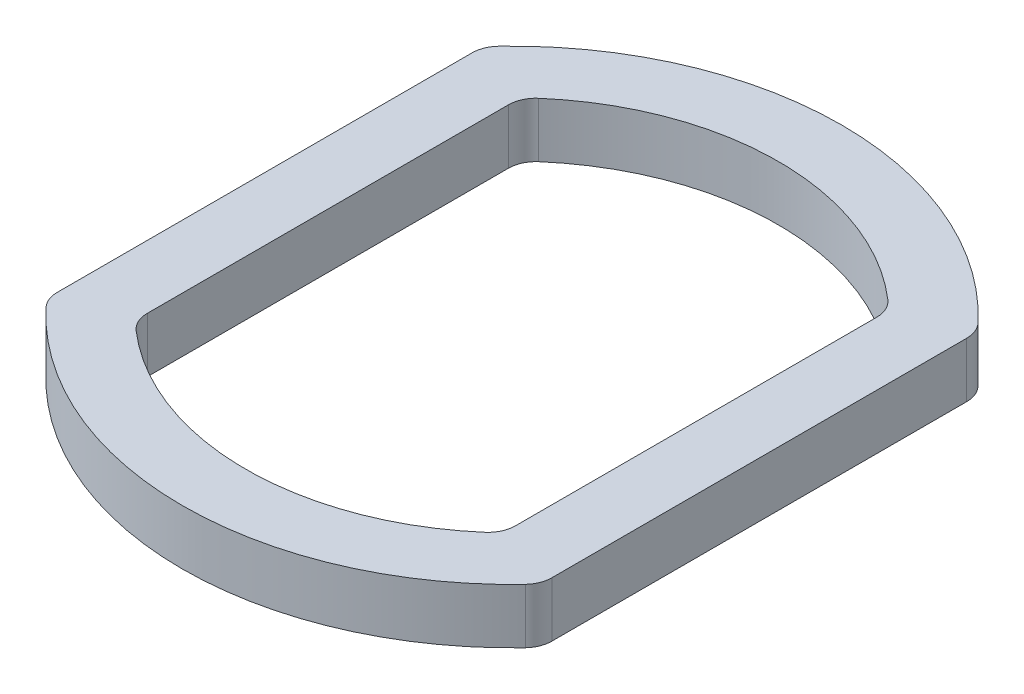
SolidWorks part; units mm, degrees
material "标准件"
ref_plane "前视基准面" through (0, 0, 0) normal (0, 0, 1) x (1, 0, 0)
ref_plane "上视基准面" through (0, 0, 0) normal (0, 1, 0) x (1, 0, 0)
ref_plane "右视基准面" through (0, 0, 0) normal (1, 0, 0) x (0, 0, -1)
sketch "草图1" plane through (0, 0, 0) normal (0, 1, 0) x (1, 0, 0)
  line L1 (67, -70.1427) -> (67, 70.1427)
  line L2 (90, -75.4983) -> (90, 75.4983)
  line L3 (-90, 75.4983) -> (-90, -75.4983)
  line L4 (90, -75.4983) -> (90, 75.4983)
  line L5 (-90, 75.4983) -> (-90, -75.4983)
  line L6 (-67, 70.1427) -> (-67, -70.1427)
  arc A0 (67, 70.1427) -> (67, 70.1427) centre (67, 70.1427) ccw
  arc A1 (67, 70.1427) -> (-67, 70.1427) centre (0, 0) ccw
  arc A2 (-67, 70.1427) -> (-67, 70.1427) centre (-67, 70.1427) ccw
  arc A3 (-67, -70.1427) -> (-67, -70.1427) centre (-67, -70.1427) ccw
  arc A4 (-67, -70.1427) -> (67, -70.1427) centre (0, 0) ccw
  arc A5 (67, -70.1427) -> (67, -70.1427) centre (67, -70.1427) ccw
  arc A6 (87.2727, 82.3618) -> (-87.2727, 82.3618) centre (0, 0) ccw
  arc A7 (90, 75.4983) -> (87.2727, 82.3618) centre (80, 75.4983) ccw
  arc A8 (87.2727, -82.3618) -> (90, -75.4983) centre (80, -75.4983) ccw
  arc A9 (-87.2727, -82.3618) -> (87.2727, -82.3618) centre (0, 0) ccw
  arc A10 (-90, -75.4983) -> (-87.2727, -82.3618) centre (-80, -75.4983) ccw
  arc A11 (-87.2727, 82.3618) -> (-90, 75.4983) centre (-80, 75.4983) ccw
  arc A12 (87.2727, 82.3618) -> (-87.2727, 82.3618) centre (0, 0) ccw
  arc A13 (90, 75.4983) -> (87.2727, 82.3618) centre (80, 75.4983) ccw
  arc A14 (87.2727, -82.3618) -> (90, -75.4983) centre (80, -75.4983) ccw
  arc A15 (-87.2727, -82.3618) -> (87.2727, -82.3618) centre (0, 0) ccw
  arc A16 (-90, -75.4983) -> (-87.2727, -82.3618) centre (-80, -75.4983) ccw
  arc A17 (-87.2727, 82.3618) -> (-90, 75.4983) centre (-80, 75.4983) ccw
  dimension "D1" = 0
  dimension "D2" = 23
extrude "凸台-拉伸1" add sketch "草图1" along normal blind 20
fillet "圆角1" radius 10 4 edges at (67, 10, -70.1427) (-67, 10, 70.1427) (67, 10, 70.1427) (-67, 10, -70.1427)
